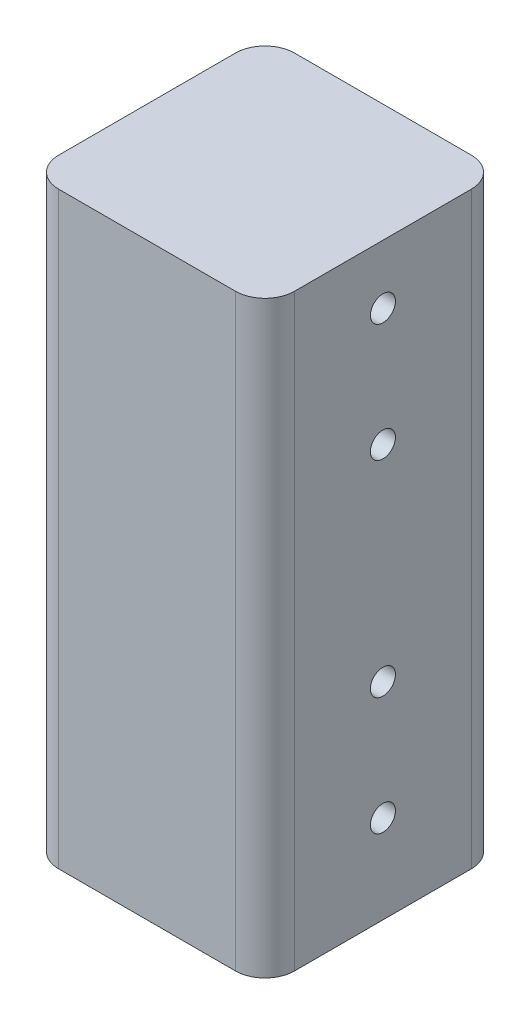
SolidWorks part; units mm, degrees
ref_plane "Front Plane" through (0, 0, 0) normal (0, 0, 1) x (1, 0, 0)
ref_plane "Top Plane" through (0, 0, 0) normal (0, 1, 0) x (1, 0, 0)
ref_plane "Right Plane" through (0, 0, 0) normal (1, 0, 0) x (0, 0, -1)
ref_plane "Plane4" through (0, 0, -30) normal (0, 0, -1) x (-1, 0, 0)
sketch "Sketch1" plane through (0, 0, -30) normal (0, 0, -1) x (-1, 0, 0)
  line L0 (-40, 0) -> (40, 0)
  line L1 (40, 0) -> (40, 199.7)
  line L2 (40, 199.7) -> (-40, 199.7)
  line L3 (-40, 199.7) -> (-40, 0)
  dimension "D1" = 80
  dimension "D2" = 199.7
extrude "Boss-Extrude1" add sketch "Sketch1" against normal blind 80
hole_wizard "Ø8.5 (8.5) Diameter Hole1" positions "Sketch4" profile "Sketch3" hole size "Ø8.5" standard "ANSI Metric"
sketch "Sketch4" plane through (40, 0, 0) normal (1, 0, 0) x (0, 0, -1)
  line L2 (-50, 199.7) -> (30, 199.7) construction
  line L3 (30, 199.7) -> (30, 0) construction
  line L4 (-50, 0) -> (30, 0) construction
  point P0 (-10, 30)
  point P1 (-10, 179.7)
  point P2 (-10, 70)
  dimension "D1" = 20
  dimension "D2" = 40
  dimension "D3" = 40
  dimension "D4" = 40
  dimension "D5" = 40
  dimension "D6" = 30
sketch "Sketch3" plane through (40, 30, 10) normal (0, 1, 0) x (0, 0, -1)
  line L0 (0, 0) -> (0, 22.5537)
  line L1 (0, 22.5537) -> (4.25, 20)
  line L2 (4.25, 20) -> (4.25, 0)
  line L5 (4.25, 0) -> (0, 0)
  line L10 (0, 22.5537) -> (-4.25, 20) construction
  line L11 (0, -6.35) -> (0, 107.95) construction
  dimension "孔直径" = 8.5
  dimension "孔深度" = 20
  dimension "导头角度" = 118
fillet "Fillet2" radius 10 4 edges at (40, 99.85, 50) (-40, 99.85, 50) (40, 99.85, -30) (-40, 99.85, -30)
sketch "Sketch5" plane through (0, 0, 0) normal (0, -1, 0) x (1, 0, 0)
  line L0 (-960, 10) -> (49040, 10) construction
  line L1 (40, 40) -> (40, -20) construction
  line L2 (0, -950) -> (0, 49050) construction
  line L3 (30, 50) -> (-30, 50) construction
  circle A0 centre (0, 10) radius 13
  point P5 (40, 10)
  point P10 (0, 50)
  dimension "D1" = 26
extrude "Cut-Extrude1" cut sketch "Sketch5" against normal blind 100
hole_wizard "Ø8.5 (8.5) Diameter Hole2" positions "Sketch6" profile "Sketch7" hole size "Ø8.5" standard "ANSI Metric"
sketch "Sketch6" plane through (40, 0, 0) normal (1, 0, 0) x (0, 0, -1)
  line L0 (30, 199.7) -> (30, 0) construction
  line L1 (-40, 199.7) -> (20, 199.7) construction
  point P0 (-10, 139.7)
  dimension "D1" = 40
  dimension "D2" = 60
sketch "Sketch7" plane through (40, 139.7, 10) normal (0, 1, 0) x (0, 0, -1)
  line L0 (0, 0) -> (0, 22.5537)
  line L1 (0, 22.5537) -> (4.25, 20)
  line L2 (4.25, 20) -> (4.25, 0)
  line L5 (4.25, 0) -> (0, 0)
  line L10 (0, 22.5537) -> (-4.25, 20) construction
  line L11 (0, -6.35) -> (0, 107.95) construction
  dimension "孔直径" = 8.5
  dimension "孔深度" = 20
  dimension "导头角度" = 118
